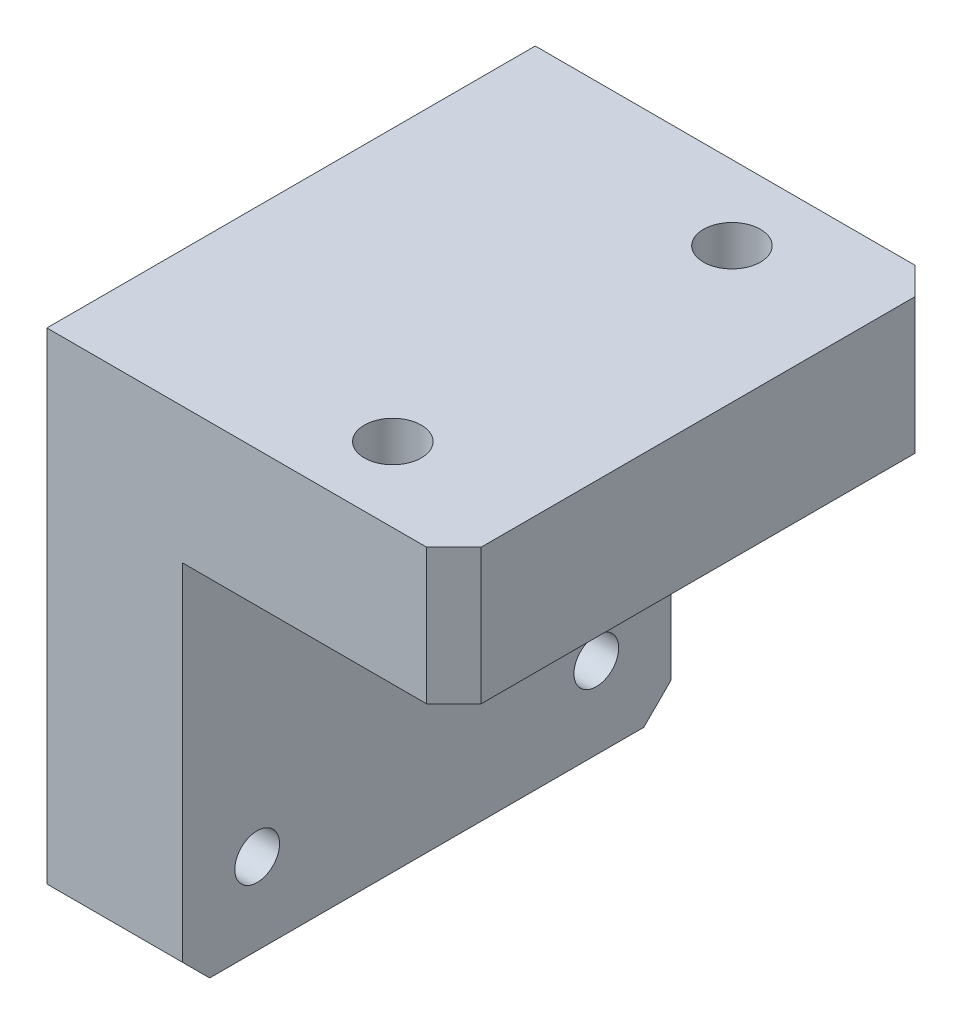
SolidWorks part; units mm, degrees
ref_plane "前视基准面" through (0, 0, 0) normal (0, 0, 1) x (1, 0, 0)
ref_plane "上视基准面" through (0, 0, 0) normal (0, 1, 0) x (1, 0, 0)
ref_plane "右视基准面" through (0, 0, 0) normal (1, 0, 0) x (0, 0, -1)
sketch "草图1" plane through (0, 0, 0) normal (0, 0, 1) x (1, 0, 0)
  line L0 (0, 0) -> (0, 37.5)
  line L1 (0, 37.5) -> (30, 37.5)
  dimension "D1" = 37.5
  dimension "D2" = 30
extrude "拉伸-薄壁1" add sketch "草图1" along normal mid plane 36 thin
chamfer "倒角1" distance 2 angle 45 4 edges at (5, 0, 18) (30, 32.5, 18) (30, 32.5, -18) (5, 0, -18)
sketch "草图4" plane through (0, 0, 0) normal (-1, 0, 0) x (0, 0, 1)
  point P0 (12.5, 27)
  point P3 (12.5, 6)
  point P6 (-12.5, 6)
  point P9 (-12.5, 27)
hole_wizard "M4 螺纹孔1" positions "草图4" profile "草图3" tap size "M4" standard "GB"
sketch "草图3" plane through (0, 27, 12.5) normal (0, 1, 0) x (0, 0, 1)
  line L0 (0, 0) -> (0, 11.0914)
  line L1 (0, 11.0914) -> (1.65, 10.1)
  line L2 (1.65, 10.1) -> (1.65, 0)
  line L5 (1.65, 0) -> (0, 0)
  line L10 (0, 11.0914) -> (-1.65, 10.1) construction
  line L11 (0, -6.35) -> (0, 107.95) construction
  dimension "螺纹孔钻头直径" = 3.3
  dimension "螺纹孔钻头深度" = 10.1
  dimension "导头角度" = 118
cosmetic thread "孔螺纹线1" parameters "D1"=8, "D2"=4
cosmetic thread "孔螺纹线2" parameters "D1"=8, "D2"=4
cosmetic thread "孔螺纹线3" parameters "D1"=8, "D2"=4
cosmetic thread "孔螺纹线4" parameters "D1"=8, "D2"=4
sketch "草图7" plane through (0, 27.5, 0) normal (0, -1, 0) x (-1, 0, 0)
  line L1 (0, 0) -> (-26.248, 0) construction
  line L3 (-30, -16) -> (-30, 16) construction
  point P0 (-20, 12.5)
  point P2 (-20, -12.5)
  dimension "D1" = 25
  dimension "D2" = 10
hole_wizard "M5 螺纹孔1" positions "草图7" profile "草图6" tap size "M5" standard "GB"
sketch "草图6" plane through (20, 27.5, -12.5) normal (1, 0, 0) x (0, 0, -1)
  line L0 (0, 0) -> (0, 13.6618)
  line L1 (0, 13.6618) -> (2.1, 12.4)
  line L2 (2.1, 12.4) -> (2.1, 0)
  line L5 (2.1, 0) -> (0, 0)
  line L10 (0, 13.6618) -> (-2.1, 12.4) construction
  line L11 (0, -6.35) -> (0, 107.95) construction
  dimension "螺纹孔钻头直径" = 4.2
  dimension "螺纹孔钻头深度" = 12.4
  dimension "导头角度" = 118
cosmetic thread "孔螺纹线5" parameters "D1"=10, "D2"=5
cosmetic thread "孔螺纹线6" parameters "D1"=10, "D2"=5
